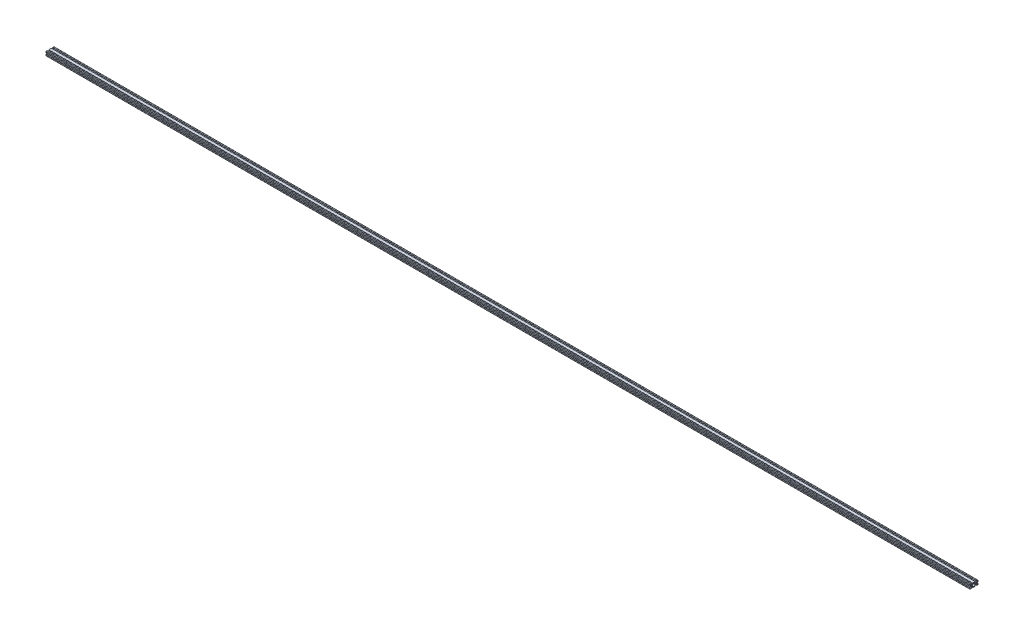
SolidWorks part; units mm, degrees
material "6063-T5"
ref_plane "Front Plane" through (0, 0, 0) normal (0, 0, 1) x (1, 0, 0)
ref_plane "Top Plane" through (0, 0, 0) normal (0, 1, 0) x (1, 0, 0)
ref_plane "Right Plane" through (0, 0, 0) normal (1, 0, 0) x (0, 0, -1)
sketch "Sketch2" plane through (0, 0, 0) normal (0, 0, 1) x (1, 0, 0)
  line L0 (-2530.1556, -1602.1869) -> (2015.8444, -1602.1869)
  dimension "D1" = 4546
other "Aluminum profile 20 X 40 X R1.5(1)"
ref_plane "Plane1" through (-2530.1556, -1602.1869, 0) normal (1, 0, 0) x (0, 1, 0)
sketch "Sketch1" plane through (-2530.1556, -1602.1869, 0) normal (1, 0, 0) x (0, 1, 0)
  line L0 (-3.6, 10) -> (-3.6, 9.5)
  line L1 (-3.6, 9.5) -> (-3.1, 9.5)
  line L2 (-3.1, 9.5) -> (-3.1, 8.5)
  line L3 (-3.1, 8.5) -> (-5.5, 8.5)
  line L4 (8.85, -10) -> (2.75, -3.9)
  line L5 (-10, -16.4) -> (-10, -3.6)
  line L6 (8.5, 10) -> (3.6, 10)
  line L7 (10, 8.5) -> (10, 3.6)
  line L8 (0, 14.8756) -> (0, 0) construction
  line L9 (0, 0) -> (10, 0) construction
  line L10 (-5.5, 8.5) -> (-5.5, 6.65)
  line L11 (-5.5, 6.65) -> (-2.75, 3.9)
  line L12 (-2.75, 3.9) -> (2.75, 3.9)
  line L13 (5.5, 6.65) -> (2.75, 3.9)
  line L14 (5.5, 8.5) -> (5.5, 6.65)
  line L15 (3.1, 8.5) -> (5.5, 8.5)
  line L16 (3.1, 9.5) -> (3.1, 8.5)
  line L17 (3.6, 9.5) -> (3.1, 9.5)
  line L18 (3.6, 10) -> (3.6, 9.5)
  line L19 (-3.6, 10) -> (-8.5, 10)
  line L20 (10, 3.6) -> (9.5, 3.6)
  line L21 (9.5, 3.6) -> (9.5, 3.1)
  line L22 (9.5, 3.1) -> (8.5, 3.1)
  line L23 (8.5, 3.1) -> (8.5, 5.5)
  line L24 (8.5, 5.5) -> (6.65, 5.5)
  line L25 (6.65, 5.5) -> (3.9, 2.75)
  line L26 (3.9, 2.75) -> (3.9, -2.75)
  line L27 (6.65, -5.5) -> (3.9, -2.75)
  line L28 (8.5, -5.5) -> (6.65, -5.5)
  line L29 (8.5, -3.1) -> (8.5, -5.5)
  line L30 (9.5, -3.1) -> (8.5, -3.1)
  line L31 (9.5, -3.6) -> (9.5, -3.1)
  line L32 (10, -3.6) -> (9.5, -3.6)
  line L33 (8.85, -10) -> (2.75, -16.1)
  line L34 (-8.85, -10) -> (-2.75, -16.1)
  line L35 (-8.85, -10) -> (-2.75, -3.9)
  line L39 (2.75, -3.9) -> (-2.75, -3.9)
  line L46 (-10, -3.6) -> (-9.5, -3.6)
  line L47 (-9.5, -3.6) -> (-9.5, -3.1)
  line L48 (-9.5, -3.1) -> (-8.5, -3.1)
  line L49 (-8.5, -3.1) -> (-8.5, -5.5)
  line L50 (-8.5, -5.5) -> (-6.65, -5.5)
  line L51 (-6.65, -5.5) -> (-3.9, -2.75)
  line L52 (-3.9, -2.75) -> (-3.9, 2.75)
  line L53 (-6.65, 5.5) -> (-3.9, 2.75)
  line L54 (-8.5, 5.5) -> (-6.65, 5.5)
  line L55 (-8.5, 3.1) -> (-8.5, 5.5)
  line L56 (-9.5, 3.1) -> (-8.5, 3.1)
  line L57 (-9.5, 3.6) -> (-9.5, 3.1)
  line L58 (-10, 3.6) -> (-9.5, 3.6)
  line L60 (-10, 3.6) -> (-10, 8.5)
  line L61 (10, -3.6) -> (10, -16.4)
  line L66 (-8.5, -30) -> (-3.6, -30)
  line L67 (-10, -28.5) -> (-10, -23.6)
  line L72 (-2.75, -16.1) -> (2.75, -16.1)
  line L80 (10, -16.4) -> (9.5, -16.4)
  line L81 (9.5, -16.4) -> (9.5, -16.9)
  line L82 (9.5, -16.9) -> (8.5, -16.9)
  line L83 (8.5, -16.9) -> (8.5, -14.5)
  line L84 (8.5, -14.5) -> (6.65, -14.5)
  line L85 (6.65, -14.5) -> (3.9, -17.25)
  line L86 (3.9, -17.25) -> (3.9, -22.75)
  line L87 (6.65, -25.5) -> (3.9, -22.75)
  line L88 (8.5, -25.5) -> (6.65, -25.5)
  line L89 (8.5, -23.1) -> (8.5, -25.5)
  line L90 (9.5, -23.1) -> (8.5, -23.1)
  line L91 (9.5, -23.6) -> (9.5, -23.1)
  line L92 (10, -23.6) -> (9.5, -23.6)
  line L93 (3.6, -30) -> (3.6, -29.5)
  line L94 (3.6, -29.5) -> (3.1, -29.5)
  line L95 (3.1, -29.5) -> (3.1, -28.5)
  line L96 (3.1, -28.5) -> (5.5, -28.5)
  line L97 (5.5, -28.5) -> (5.5, -26.65)
  line L98 (5.5, -26.65) -> (2.75, -23.9)
  line L99 (2.75, -23.9) -> (-2.75, -23.9)
  line L100 (-5.5, -26.65) -> (-2.75, -23.9)
  line L101 (-5.5, -28.5) -> (-5.5, -26.65)
  line L102 (-3.1, -28.5) -> (-5.5, -28.5)
  line L103 (-3.1, -29.5) -> (-3.1, -28.5)
  line L104 (-3.6, -29.5) -> (-3.1, -29.5)
  line L105 (-3.6, -30) -> (-3.6, -29.5)
  line L106 (-10, -23.6) -> (-9.5, -23.6)
  line L107 (-9.5, -23.6) -> (-9.5, -23.1)
  line L108 (-9.5, -23.1) -> (-8.5, -23.1)
  line L109 (-8.5, -23.1) -> (-8.5, -25.5)
  line L110 (-8.5, -25.5) -> (-6.65, -25.5)
  line L111 (-6.65, -25.5) -> (-3.9, -22.75)
  line L112 (-3.9, -22.75) -> (-3.9, -17.25)
  line L113 (-6.65, -14.5) -> (-3.9, -17.25)
  line L114 (-8.5, -14.5) -> (-6.65, -14.5)
  line L115 (-8.5, -16.9) -> (-8.5, -14.5)
  line L116 (-9.5, -16.9) -> (-8.5, -16.9)
  line L117 (-9.5, -16.4) -> (-9.5, -16.9)
  line L118 (-10, -16.4) -> (-9.5, -16.4)
  line L119 (3.6, -30) -> (8.5, -30)
  line L121 (10, -23.6) -> (10, -28.5)
  line L122 (0, -20) -> (10, -20) construction
  line L125 (3.6, -10) -> (3.6, -9.5) [skipped]
  line L127 (3.6, -9.5) -> (3.1, -9.5) [skipped]
  line L129 (3.1, -9.5) -> (3.1, -8.5) [skipped]
  line L131 (3.1, -8.5) -> (5.5, -8.5) [skipped]
  line L133 (-3.1, -8.5) -> (-5.5, -8.5) [skipped]
  line L135 (-3.1, -9.5) -> (-3.1, -8.5) [skipped]
  line L137 (-3.6, -9.5) -> (-3.1, -9.5) [skipped]
  line L139 (-3.6, -10) -> (-3.6, -9.5) [skipped]
  line L141 (-3.6, -10) -> (-3.6, -10.5) [skipped]
  line L142 (-3.6, -10.5) -> (-3.1, -10.5) [skipped]
  line L143 (-3.1, -10.5) -> (-3.1, -11.5) [skipped]
  line L144 (-3.1, -11.5) -> (-5.5, -11.5) [skipped]
  line L145 (8.5, -10) -> (3.6, -10) [skipped]
  line L146 (3.1, -11.5) -> (5.5, -11.5) [skipped]
  line L147 (3.1, -10.5) -> (3.1, -11.5) [skipped]
  line L148 (3.6, -10.5) -> (3.1, -10.5) [skipped]
  line L149 (3.6, -10) -> (3.6, -10.5) [skipped]
  line L150 (-3.6, -10) -> (-8.5, -10) [skipped]
  line L151 (-10, -16.4) -> (-10, -11.5) [skipped]
  line L152 (10, -11.5) -> (10, -16.4) [skipped]
  line L154 (-5.5, -8.5) -> (-5.5, -6.65) [skipped]
  line L156 (5.5, -8.5) -> (5.5, -6.65) [skipped]
  line L157 (5.5, -11.5) -> (5.5, -13.35) [skipped]
  line L158 (-5.5, -11.5) -> (-5.5, -13.35) [skipped]
  line L160 (-12.2446, -13.3946) -> (-10, -11.15) [skipped]
  line L161 (13.644, -5.206) -> (10, -8.85) [skipped]
  line L163 (12.1963, -13.3463) -> (10, -11.15) [skipped]
  line L164 (-11.1344, -7.7156) -> (-10, -8.85) [skipped]
  circle A0 centre (0, 0) radius 2.5
  arc A1 (-10, 8.5) -> (-8.5, 10) centre (-8.5, 8.5) cw
  arc A2 (10, 8.5) -> (8.5, 10) centre (8.5, 8.5) ccw
  arc A3 (10, -28.5) -> (8.5, -30) centre (8.5, -28.5) cw
  arc A4 (-10, -28.5) -> (-8.5, -30) centre (-8.5, -28.5) ccw
  circle A5 centre (0, -20) radius 2.5
  arc A12 (-10, -11.5) -> (-8.5, -10) centre (-8.5, -11.5) cw [skipped]
  arc A13 (10, -11.5) -> (8.5, -10) centre (8.5, -11.5) ccw [skipped]
  point P0 (-10, 0)
  point P1 (10, 0)
  point P2 (0, 10)
  point P4 (0, 0)
  point P5 (0, -10)
  point P6 (-10, -10)
  point P7 (10, 10)
  point P8 (-10, 10)
  point P12 (-10, -10)
  point P13 (10, -10)
  point P15 (0, -10)
  point P16 (10, -10)
  point P36 (-10, 10)
  point P39 (10, 10)
  point P43 (-10, -20)
  point P44 (10, -20)
  point P62 (0, 0)
  point P88 (0, -30)
  point P89 (0, -20)
  point P90 (-10, -30)
  point P91 (10, -30)
  dimension "D1" = 11
  dimension "D2" = 20
  dimension "D3" = 6.2
  dimension "D4" = 7.2
  dimension "D5" = 6.1
  dimension "D6" = 5
  dimension "D7" = 1.5
  dimension "D8" = 45
  dimension "D14" = 20
  dimension "D15" = 1.5
  dimension "D9" = 0.5
  dimension "D10" = 1
  dimension "D11" = 5.5
  dimension "D12" = 10
  dimension "D13" = 40
  dimension "D16" = 45
  dimension "D17" = 45
  dimension "D18" = 45
  dimension "D19" = 6.2
hole_wizard "M6 Tapped Hole1" positions "Sketch4" profile "Sketch3" tap size "M6" standard "GB"
sketch "Sketch4" plane through (2015.8444, 0, 0) normal (1, 0, 0) x (0, 0, -1)
  point P0 (0, -1602.1869)
  point P3 (20, -1602.1869)
sketch "Sketch3" plane through (2015.8444, -1602.1869, 0) normal (0, 1, 0) x (0, 0, -1)
  line L0 (0, 0) -> (0, 16.5022)
  line L1 (0, 16.5022) -> (2.5, 15)
  line L2 (2.5, 15) -> (2.5, 0)
  line L5 (2.5, 0) -> (0, 0)
  line L10 (0, 16.5022) -> (-2.5, 15) construction
  line L11 (0, -6.35) -> (0, 107.95) construction
  dimension "螺纹孔钻头直径" = 5
  dimension "螺纹孔钻头深度" = 15
  dimension "导头角度" = 118
